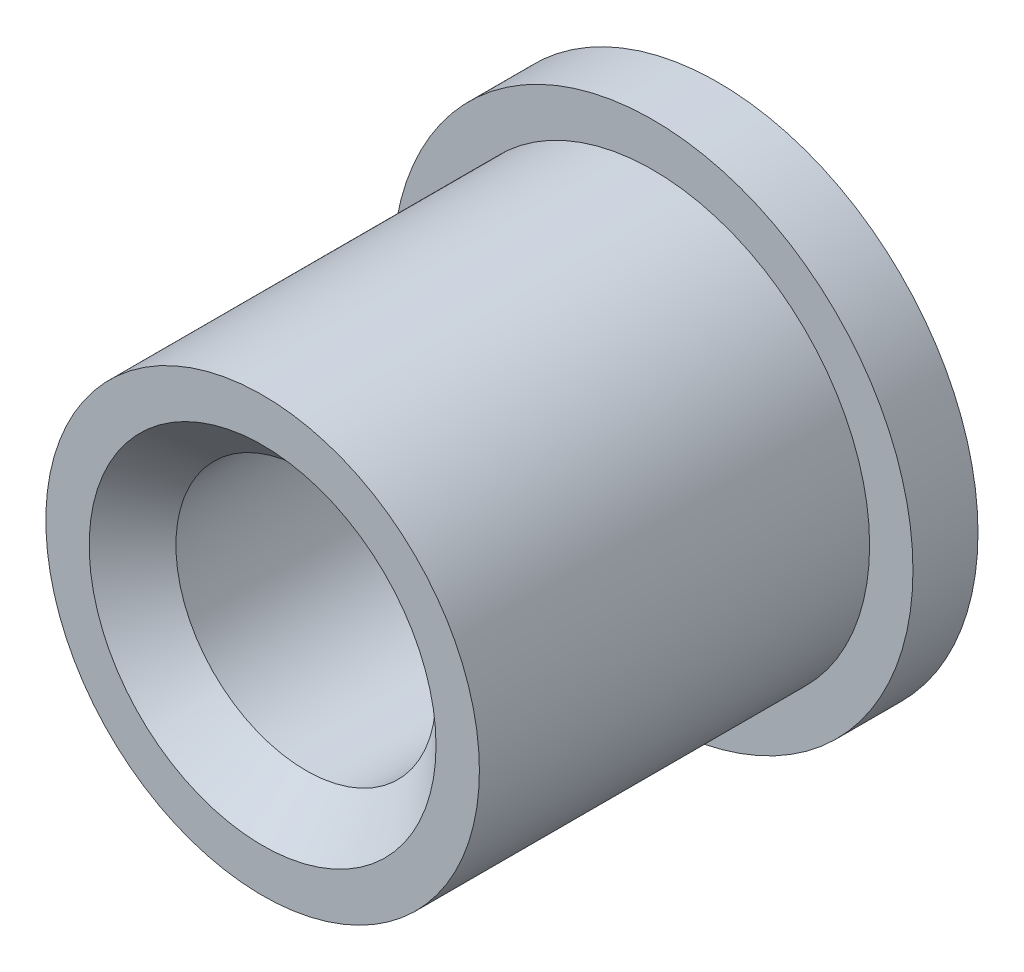
from build123d import *

# Parameters (mm, degrees)
SKETCH1_R           = 12
BOSS_EXTRUDE1_DEPTH = 3
SKETCH2_R           = 10
BOSS_EXTRUDE2_DEPTH = 18
SKETCH3_R           = 6
CUT_EXTRUDE1_DEPTH  = 26
CHAMFER1_SIZE       = 2


with BuildPart() as part:
    # Sketch1 → Boss-Extrude1 (new body)
    with BuildSketch(Plane.XY):
        Circle(SKETCH1_R)
    extrude(amount=BOSS_EXTRUDE1_DEPTH)

    # Sketch2 → Boss-Extrude2 (add)
    with BuildSketch(Plane.XY.offset(3)):
        Circle(SKETCH2_R)
    extrude(amount=BOSS_EXTRUDE2_DEPTH)

    # Sketch3 → Cut-Extrude1 (cut)
    with BuildSketch(Plane.XY.offset(21)):
        Circle(SKETCH3_R)
    extrude(amount=-CUT_EXTRUDE1_DEPTH, mode=Mode.SUBTRACT)

    # Chamfer1
    chamfer1_edges = [part.edges().sort_by_distance(p)[0] for p in [
        (-6, 0, 21),
    ]]
    chamfer(chamfer1_edges, length=CHAMFER1_SIZE)


solid = part.part
